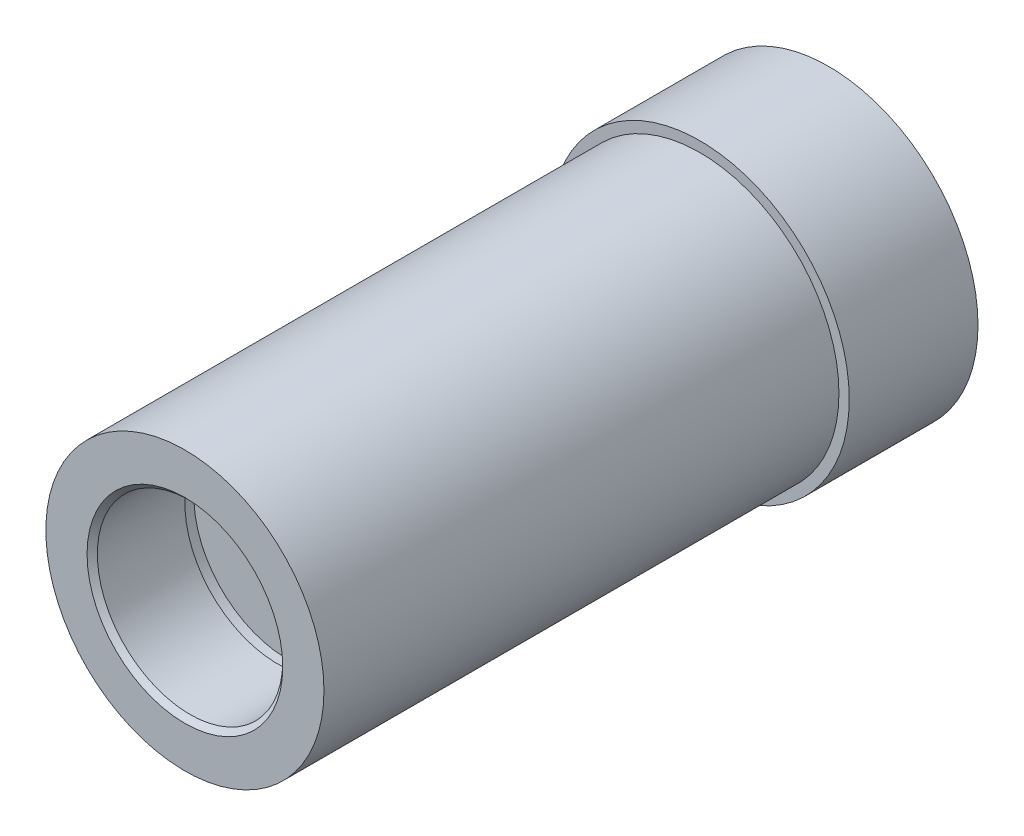
SolidWorks part; units mm, degrees
ref_plane "Front Plane" through (0, 0, 0) normal (0, 0, 1) x (1, 0, 0)
ref_plane "Top Plane" through (0, 0, 0) normal (0, 1, 0) x (1, 0, 0)
ref_plane "Right Plane" through (0, 0, 0) normal (1, 0, 0) x (0, 0, -1)
sketch "Sketch1" plane through (0, 0, 0) normal (0, 0, 1) x (1, 0, 0)
  circle A0 centre (0, 0) radius 29
  dimension "D1" = 58
extrude "Boss-Extrude1" add sketch "Sketch1" along normal blind 25
sketch "Sketch2" plane through (0, 0, 25) normal (0, 0, 1) x (1, 0, 0)
  circle A0 centre (0, 0) radius 27
  dimension "D1" = 54
extrude "Boss-Extrude2" add sketch "Sketch2" along normal blind 100
sketch "Sketch7" plane through (0, 0, 0) normal (0, 0, -1) x (-1, 0, 0)
  circle A0 centre (0, 0) radius 24
  dimension "D1" = 48
extrude "Cut-Extrude4" cut sketch "Sketch7" against normal blind 22
sketch "Sketch8" plane through (0, 0, 22) normal (0, 0, -1) x (-1, 0, 0)
  circle A0 centre (0, 0) radius 24.1
  dimension "D1" = 48.2
extrude "Cut-Extrude5" cut sketch "Sketch8" against normal blind 3
chamfer "Chamfer1" distance 1 angle 45 1 edges at (-24, 0, 0)
sketch "Sketch9" plane through (0, 0, 125) normal (0, 0, 1) x (1, 0, 0)
  circle A0 centre (0, 0) radius 18
  dimension "D1" = 36
extrude "Cut-Extrude6" cut sketch "Sketch9" against normal blind 18
sketch "Sketch10" plane through (0, 0, 107) normal (0, 0, 1) x (1, 0, 0)
  circle A0 centre (0, 0) radius 18.25
  dimension "D1" = 36.5
extrude "Cut-Extrude7" cut sketch "Sketch10" against normal blind 2
chamfer "Chamfer2" distance 1 angle 45 1 edges at (18, 0, 125)
